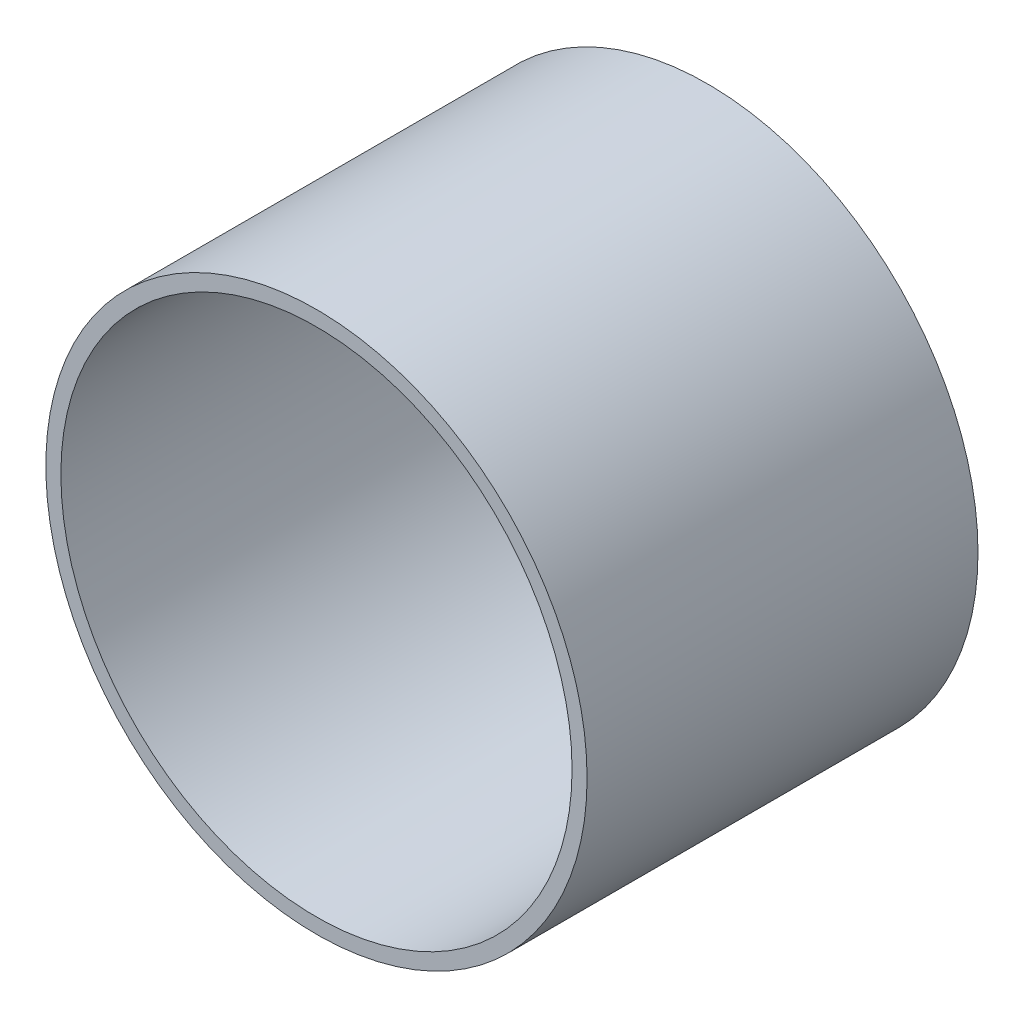
SolidWorks part; units mm, degrees
ref_plane "前视基准面" through (0, 0, 0) normal (0, 0, 1) x (1, 0, 0)
ref_plane "上视基准面" through (0, 0, 0) normal (0, 1, 0) x (1, 0, 0)
ref_plane "右视基准面" through (0, 0, 0) normal (1, 0, 0) x (0, 0, -1)
other "Configuration Table"
sketch "草图1" plane through (0, 0, 0) normal (0, 0, 1) x (1, 0, 0)
  circle A0 centre (0, 0) radius 42.5
  circle A1 centre (0, 0) radius 45
  dimension "D1" = 85
  dimension "D2" = 90
extrude "凸台-拉伸1" add sketch "草图1" along normal mid plane 65
